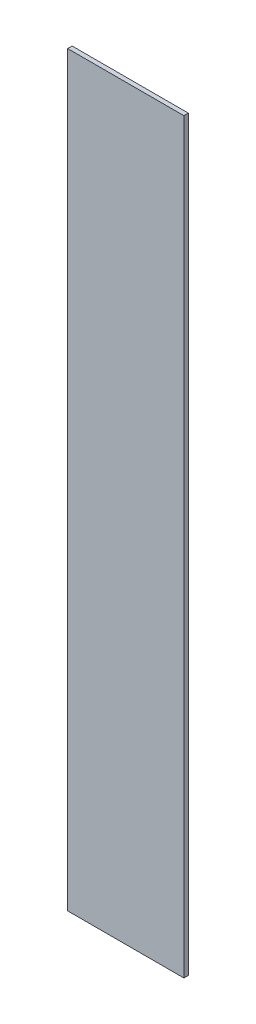
from build123d import *

# Parameters (mm, degrees)
SKETCH_1_W      = 131
SKETCH_1_H      = 842
EXTRUDE_1_DEPTH = 5


with BuildPart() as part:
    # 草图1 → 凸台-拉伸1 (new body)
    with BuildSketch(Plane.XY):
        Rectangle(SKETCH_1_W, SKETCH_1_H)
    extrude(amount=EXTRUDE_1_DEPTH)


solid = part.part
